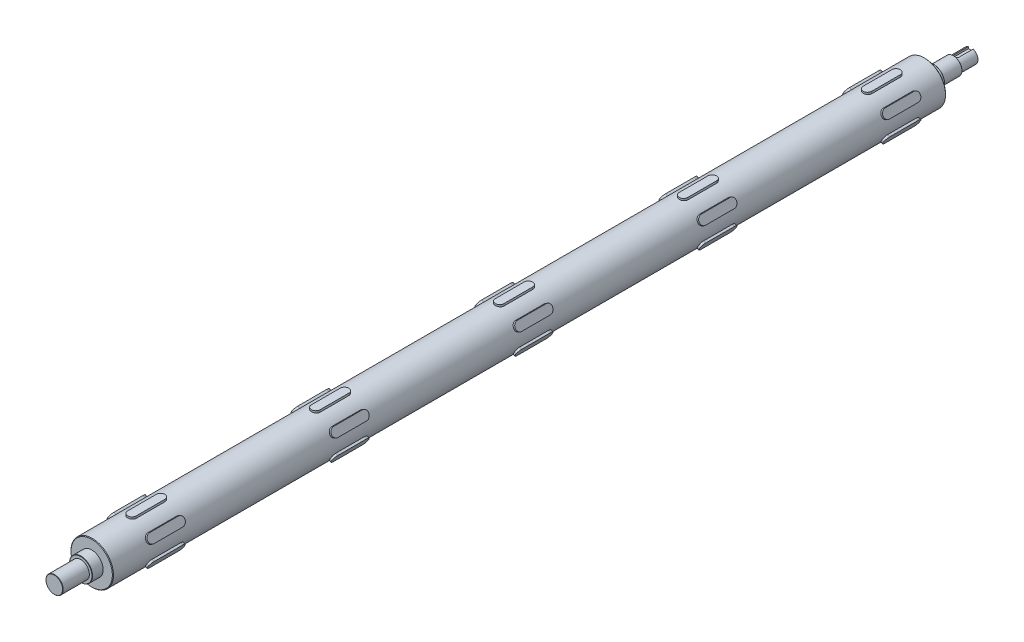
SolidWorks part; units mm, degrees
ref_plane "前视基准面" through (0, 0, 0) normal (0, 0, 1) x (1, 0, 0)
ref_plane "上视基准面" through (0, 0, 0) normal (0, 1, 0) x (1, 0, 0)
ref_plane "右视基准面" through (0, 0, 0) normal (1, 0, 0) x (0, 0, -1)
sketch "草图1" plane through (0, 0, 0) normal (0, 0, 1) x (1, 0, 0)
  circle A0 centre (0, 0) radius 37
  dimension "D1" = 74
extrude "凸台-拉伸1" add sketch "草图1" along normal blind 1450
sketch "草图2" plane through (0, 0, 0) normal (0, 0, -1) x (-1, 0, 0)
  circle A0 centre (0, 0) radius 20
  dimension "D1" = 40
extrude "凸台-拉伸2" add sketch "草图2" along normal blind 50
sketch "草图3" plane through (0, 0, 1450) normal (0, 0, 1) x (1, 0, 0)
  circle A0 centre (0, 0) radius 20
  dimension "D1" = 40
extrude "凸台-拉伸3" add sketch "草图3" along normal blind 45
ref_plane "基准面1" through (0, 37.5, 0) normal (0, 1, 0) x (1, 0, 0)
sketch "草图5" plane through (0, 37.5, 0) normal (0, 1, 0) x (1, 0, 0)
  line L0 (0, -100) -> (0, -50) construction
  line L1 (-7.5, -100) -> (-7.5, -50)
  line L2 (7.5, -100) -> (7.5, -50)
  line L3 (0, 0) -> (0, -196.0747) construction
  line L4 (37, 0) -> (-37, 0) construction
  arc A0 (-7.5, -100) -> (7.5, -100) centre (0, -100) ccw
  arc A1 (7.5, -50) -> (-7.5, -50) centre (0, -50) ccw
  point P2 (0, -75)
  dimension "D2" = 50
  dimension "D3" = 7.5
  dimension "D1" = 50
extrude "凸台-拉伸4" add sketch "草图5" along normal mid plane 5
pattern_linear "阵列(线性)1" count 5 spacing 320 along (0, 0, 1) of "凸台-拉伸4"
pattern_circular "阵列(圆周)1" count 6 over 360 about axis through (0, 0, 0) along (0, 0, 1) of "凸台-拉伸4", "阵列(线性)1"
chamfer "倒角1" distance 1 angle 45 2 edges at (37, 0, 0) (37, 0, 1450)
sketch "草图6" plane through (0, 0, -50) normal (0, 0, -1) x (-1, 0, 0)
  circle A0 centre (0, 0) radius 15
  dimension "D1" = 30
extrude "切除-拉伸1" cut sketch "草图6" against normal blind 35 flip side to cut
sketch "草图7" plane through (0, 0, 1495) normal (0, 0, 1) x (1, 0, 0)
  circle A0 centre (0, 0) radius 15
  dimension "D1" = 30
extrude "切除-拉伸2" cut sketch "草图7" against normal blind 26 flip side to cut
sketch "草图8" plane through (0, 0, 1495) normal (0, 0, 1) x (1, 0, 0)
  circle A1 centre (0, 0) radius 15
  circle A2 centre (0, 0) radius 15
  dimension "D1" = 0
extrude "凸台-拉伸5" add sketch "草图8" along normal blind 20
ref_plane "基准面2" through (0, 0, 732.5) normal (0, 0, -1) x (-1, 0, 0)
chamfer "倒角2" distance 0.5 angle 45 4 edges at (-15, 0, -50) (-20, 0, -15) (15, 0, 1515) (20, 0, 1469)
sketch "草图9" plane through (0, 0, -50) normal (0, 0, -1) x (-1, 0, 0)
  circle A0 centre (0, 0) radius 12.5
  dimension "D1" = 25
extrude "凸台-拉伸6" add sketch "草图9" along normal blind 30
ref_plane "基准面3" through (0, 8.5, 0) normal (0, 1, 0) x (1, 0, 0)
sketch "草图10" plane through (0, 8.5, 0) normal (0, 1, 0) x (1, 0, 0)
  line L0 (0, 80) -> (0, 55) construction
  line L1 (4, 80) -> (4, 55)
  line L2 (-4, 80) -> (-4, 55)
  line L3 (12.5, 80) -> (-12.5, 80) construction
  arc A0 (4, 80) -> (-4, 80) centre (0, 80) ccw
  arc A1 (-4, 55) -> (4, 55) centre (0, 55) ccw
  point P3 (0, 67.5)
  dimension "D1" = 25
  dimension "D2" = 8
  dimension "D3" = 0
extrude "切除-拉伸3" cut sketch "草图10" along normal blind 60
hole_wizard "M8 螺纹孔1" positions "草图11" profile "草图13" tap size "M8" standard "GB"
sketch "草图11" plane through (0, 0, -80) normal (0, 0, -1) x (-1, 0, 0)
  point P0 (0, 0)
sketch "草图13" plane through (0, 0, -80) normal (1, 0, 0) x (0, 1, 0)
  line L0 (0, 0) -> (0, 21.7929)
  line L1 (0, 21.7929) -> (3.4, 19.75)
  line L2 (3.4, 19.75) -> (3.4, 0)
  line L5 (3.4, 0) -> (0, 0)
  line L10 (0, 21.7929) -> (-3.4, 19.75) construction
  line L11 (0, -6.35) -> (0, 107.95) construction
  dimension "螺纹孔钻头直径" = 6.8
  dimension "螺纹孔钻头深度" = 19.75
  dimension "导头角度" = 118
cosmetic thread "孔螺蚊线1" parameters "D1"=16, "D2"=8
